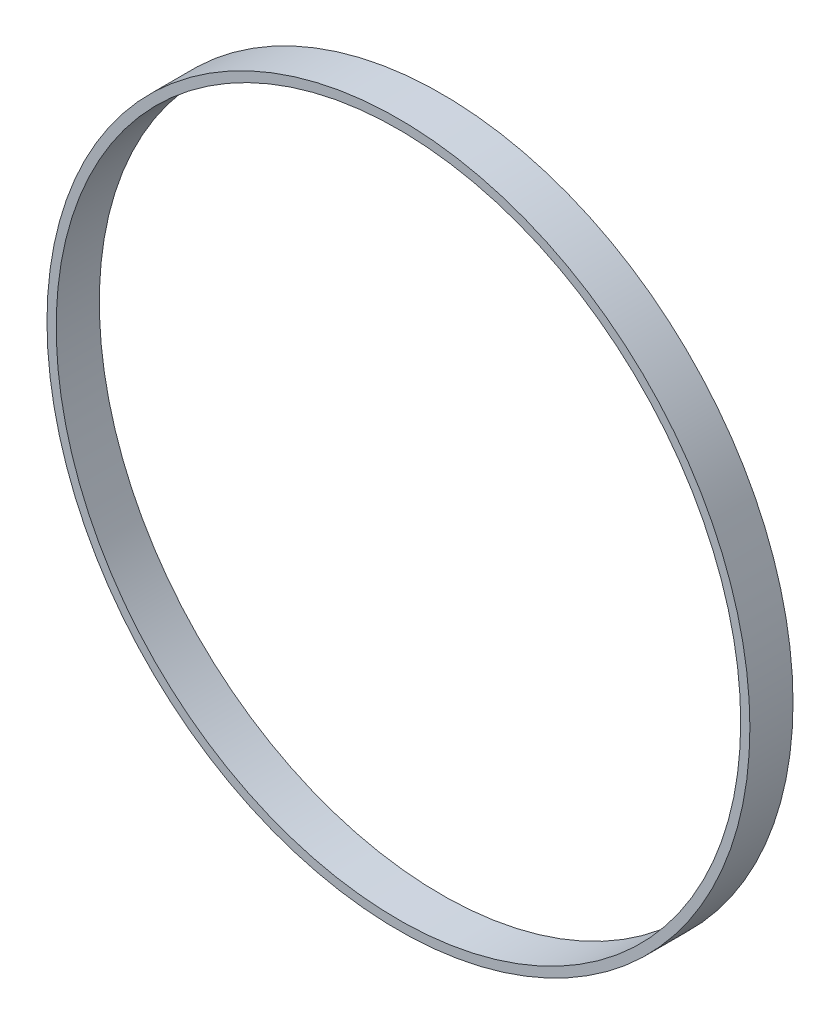
from build123d import *

# Parameters (mm, degrees)
SKETCH_1_R      = 122.25
SKETCH_1_R_2    = 119.05
EXTRUDE_1_DEPTH = 15


with BuildPart() as part:
    # 草图1 → 凸台-拉伸1 (new body)
    with BuildSketch(Plane.XY):
        Circle(SKETCH_1_R)
        Circle(SKETCH_1_R_2, mode=Mode.SUBTRACT)
    extrude(amount=EXTRUDE_1_DEPTH)


solid = part.part
